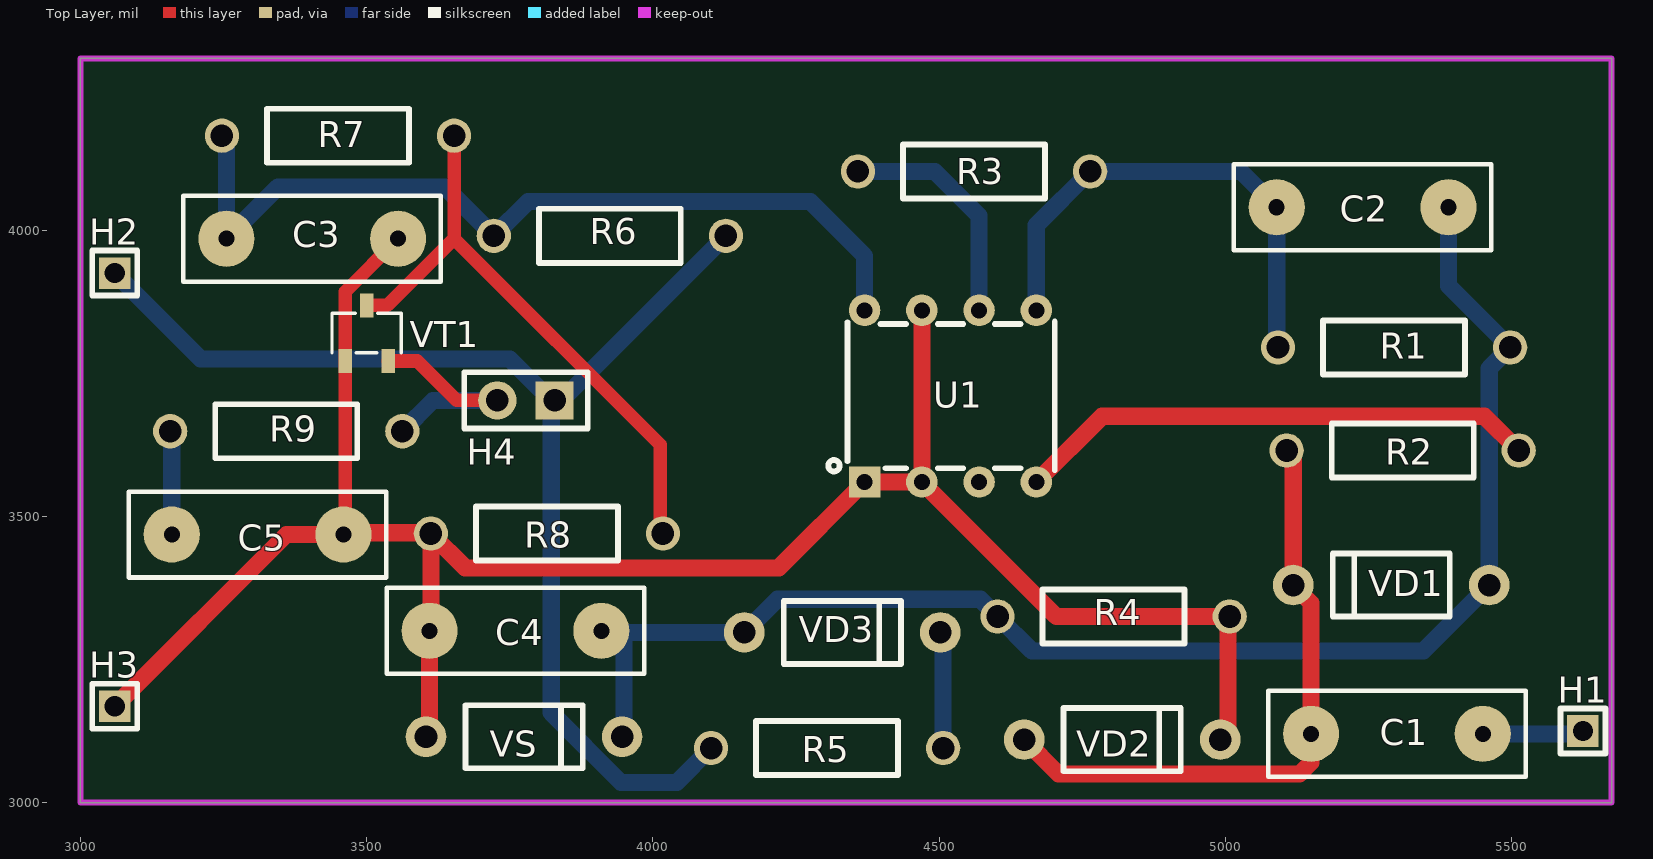
[diagram p0: Top Layer view]
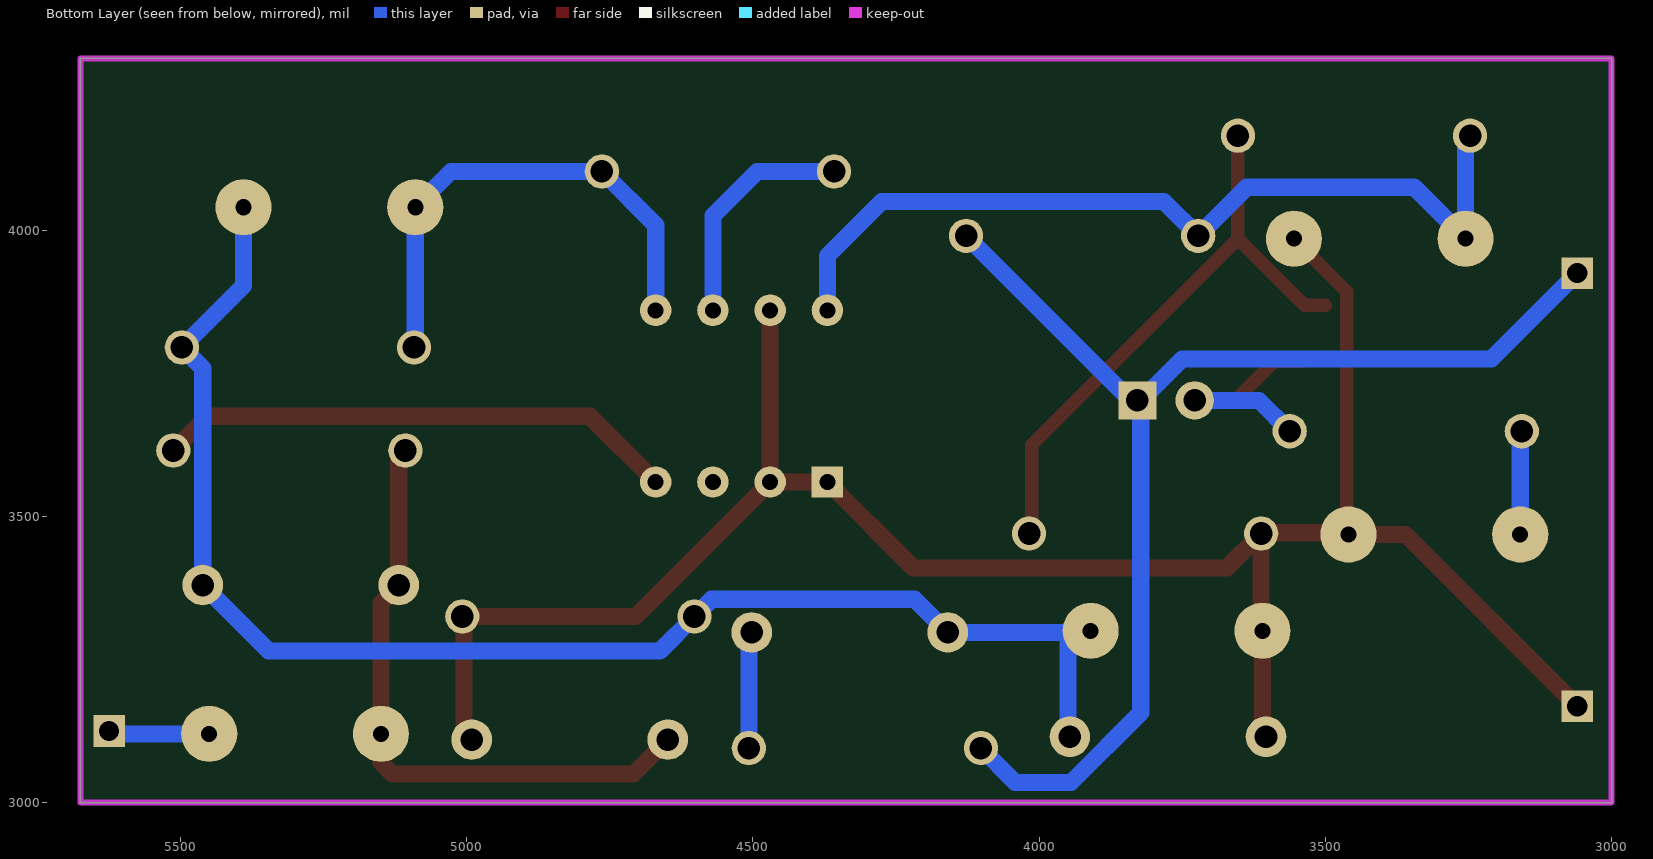
[diagram p1: Bottom Layer view, seen from below]
# Altium PCB MISC75395.pcbdoc
Units mil, origin at the board's own origin, x right, y up, seen from the top; angles counter-clockwise.
Board outline 2675 x 1300 mil, 2 copper layers (Top Layer, Bottom Layer), stack 62.206 mil thick; 24 components, 13 nets, 52 pads, 0 vias.

## Layer stack, top to bottom
Top Solder Mask Layer: solder mask 0.394, Dk 3.3
Top Layer: signal copper 1.379
Dielectric1: surface 59.449, FR4, Dk 4.5
Bottom Layer: signal copper 1.378
Bottom Solder Mask Layer: solder mask 0.394, Dk 3.3

## Board outline
3000,4300 3000,3000 5675,3000 5675,4300

## Design rules (kind name [scope] priority, off if disabled: settings)
BoardOutlineClearance copperThickness2oz_1 [All] p2 off: genericclearance=7.99 ignorepadtopadclearanceinfootprint=FALSE except(0: Arc-SplitContinuation Track-SplitContinuation SMDPad-SplitContinuation THPad-SplitContinuation Via-SplitContinuation Fill-SplitContinuation Region-SplitContinuation Poly-SplitContinuation Text-SplitContinuation Hole-SplitContinuation; 5.98: Arc-CutoutEdge Track-CutoutEdge SMDPad-CutoutEdge THPad-CutoutEdge Via-CutoutEdge Text-CutoutEdge; 6.89: Hole-OutlineEdge Hole-CutoutEdge; 10: Poly-OutlineEdge Poly-CutoutEdge; 11.81: Arc-OutlineEdge Track-OutlineEdge SMDPad-OutlineEdge THPad-OutlineEdge Via-OutlineEdge Fill-OutlineEdge Region-OutlineEdge Text-OutlineEdge Fill-CutoutEdge Region-CutoutEdge)
BoardOutlineClearance Plane_innerPlane_1 [All] p4 off: genericclearance=4.02 ignorepadtopadclearanceinfootprint=FALSE except(0: Arc-SplitContinuation Track-SplitContinuation SMDPad-SplitContinuation THPad-SplitContinuation Via-SplitContinuation Fill-SplitContinuation Region-SplitContinuation Poly-SplitContinuation Text-SplitContinuation Hole-SplitContinuation; 5.98: Arc-CutoutEdge Track-CutoutEdge SMDPad-CutoutEdge THPad-CutoutEdge Via-CutoutEdge Text-CutoutEdge; 6.89: Hole-OutlineEdge Hole-CutoutEdge; 10: Poly-OutlineEdge Poly-CutoutEdge; 11.81: Arc-OutlineEdge Track-OutlineEdge SMDPad-OutlineEdge THPad-OutlineEdge Via-OutlineEdge Fill-OutlineEdge Region-OutlineEdge Text-OutlineEdge Fill-CutoutEdge Region-CutoutEdge)
BoardOutlineClearance Copper_copperRegion_1 [All] p6 off: genericclearance=4.02 ignorepadtopadclearanceinfootprint=FALSE except(0: Arc-SplitContinuation Track-SplitContinuation SMDPad-SplitContinuation THPad-SplitContinuation Via-SplitContinuation Fill-SplitContinuation Region-SplitContinuation Poly-SplitContinuation Text-SplitContinuation Hole-SplitContinuation; 5.98: Arc-CutoutEdge Track-CutoutEdge SMDPad-CutoutEdge THPad-CutoutEdge Via-CutoutEdge Text-CutoutEdge; 6.89: Hole-OutlineEdge Hole-CutoutEdge; 10: Poly-OutlineEdge Poly-CutoutEdge; 11.81: Arc-OutlineEdge Track-OutlineEdge SMDPad-OutlineEdge THPad-OutlineEdge Via-OutlineEdge Fill-OutlineEdge Region-OutlineEdge Text-OutlineEdge Fill-CutoutEdge Region-CutoutEdge)
BoardOutlineClearance copperThickness1oz_1 [All] p8: genericclearance=4.02 ignorepadtopadclearanceinfootprint=FALSE except(0: Arc-SplitContinuation Track-SplitContinuation SMDPad-SplitContinuation THPad-SplitContinuation Via-SplitContinuation Fill-SplitContinuation Region-SplitContinuation Poly-SplitContinuation Text-SplitContinuation Hole-SplitContinuation; 5.98: Arc-CutoutEdge Track-CutoutEdge SMDPad-CutoutEdge THPad-CutoutEdge Via-CutoutEdge Text-CutoutEdge; 6.89: Hole-OutlineEdge Hole-CutoutEdge; 10: Poly-OutlineEdge Poly-CutoutEdge; 11.81: Arc-OutlineEdge Track-OutlineEdge SMDPad-OutlineEdge THPad-OutlineEdge Via-OutlineEdge Fill-OutlineEdge Region-OutlineEdge Text-OutlineEdge Fill-CutoutEdge Region-CutoutEdge)
Clearance copperThickness2oz [All] p1 off: gap=7.99 ignorepadtopadclearanceinfootprint=FALSE except(5.98: SMDPad-Track SMDPad-SMDPad THPad-Track SMDPad-THPad THPad-THPad Track-Via SMDPad-Via THPad-Via Via-Via Fill-SMDPad Region-SMDPad Fill-THPad Region-THPad Fill-Via Region-Via Fill-Fill Fill-Region Region-Region Arc-Track Arc-SMDPad Arc-THPad Arc-Via Fill-Arc Region-Arc Arc-Arc Text-Track SMDPad-Text Text-THPad Text-Via Fill-Text Region-Text Arc-Text Text-Text; 6.89: Hole-Track Hole-SMDPad Hole-THPad Hole-Via Fill-Hole Region-Hole Hole-Arc Hole-Text; 10: Poly-Track Poly-SMDPad Poly-THPad Poly-Via Poly-Fill Poly-Region Poly-Poly Poly-Arc Poly-Text Poly-Hole; 11.81: Fill-Track Region-Track)
Clearance Plane_innerPlane [All] p3 off: gap=4.02 ignorepadtopadclearanceinfootprint=FALSE except(5.98: SMDPad-Track SMDPad-SMDPad THPad-Track SMDPad-THPad THPad-THPad Track-Via SMDPad-Via THPad-Via Via-Via Fill-SMDPad Region-SMDPad Fill-THPad Region-THPad Fill-Via Region-Via Fill-Fill Fill-Region Region-Region Arc-Track Arc-SMDPad Arc-THPad Arc-Via Fill-Arc Region-Arc Arc-Arc Text-Track SMDPad-Text Text-THPad Text-Via Fill-Text Region-Text Arc-Text Text-Text; 6.89: Hole-Track Hole-SMDPad Hole-THPad Hole-Via Fill-Hole Region-Hole Hole-Arc Hole-Text; 10: Poly-Track Poly-SMDPad Poly-THPad Poly-Via Poly-Fill Poly-Region Poly-Poly Poly-Arc Poly-Text Poly-Hole; 11.81: Fill-Track Region-Track)
Clearance Copper_copperRegion [All] p5 off: gap=4.02 ignorepadtopadclearanceinfootprint=FALSE except(5.98: SMDPad-Track SMDPad-SMDPad THPad-Track SMDPad-THPad THPad-THPad Track-Via SMDPad-Via THPad-Via Via-Via Fill-SMDPad Region-SMDPad Fill-THPad Region-THPad Fill-Via Region-Via Fill-Fill Fill-Region Region-Region Arc-Track Arc-SMDPad Arc-THPad Arc-Via Fill-Arc Region-Arc Arc-Arc Text-Track SMDPad-Text Text-THPad Text-Via Fill-Text Region-Text Arc-Text Text-Text; 6.89: Hole-Track Hole-SMDPad Hole-THPad Hole-Via Fill-Hole Region-Hole Hole-Arc Hole-Text; 10: Poly-Track Poly-SMDPad Poly-THPad Poly-Via Poly-Fill Poly-Region Poly-Poly Poly-Arc Poly-Text Poly-Hole; 11.81: Fill-Track Region-Track)
Clearance copperThickness1oz [All] p7: gap=4.02 ignorepadtopadclearanceinfootprint=FALSE except(5.98: SMDPad-Track SMDPad-SMDPad THPad-Track SMDPad-THPad THPad-THPad Track-Via SMDPad-Via THPad-Via Via-Via Fill-SMDPad Region-SMDPad Fill-THPad Region-THPad Fill-Via Region-Via Fill-Fill Fill-Region Region-Region Arc-Track Arc-SMDPad Arc-THPad Arc-Via Fill-Arc Region-Arc Arc-Arc Text-Track SMDPad-Text Text-THPad Text-Via Fill-Text Region-Text Arc-Text Text-Text; 6.89: Hole-Track Hole-SMDPad Hole-THPad Hole-Via Fill-Hole Region-Hole Hole-Arc Hole-Text; 10: Poly-Track Poly-SMDPad Poly-THPad Poly-Via Poly-Fill Poly-Region Poly-Poly Poly-Arc Poly-Text Poly-Hole; 11.81: Fill-Track Region-Track)
DiffPairsRouting differentialPair [All] p1: maxlimit=6 minlimit=6 mostfreqgap=6 toplayer_minwidth=5 toplayer_prefwidth=10 toplayer_maxwidth=100 toplayer_mingap=6 toplayer_prefgap=6 toplayer_maxgap=6 bottomlayer_minwidth=5 bottomlayer_prefwidth=10 bottomlayer_maxwidth=100 bottomlayer_mingap=6 bottomlayer_prefgap=6 bottomlayer_maxgap=6 maxuncoupledlength=10
HoleToHoleClearance otherClearance [All] p1: gap=11.81 allowstackedmicrovias=TRUE
Length netLength [All] p1: minlimit=0 maxlimit=0
PasteMaskExpansion pasteMaskExpansion [All] p1: expansion=0
PlaneConnect innerPlane [All] p1: planeconnectstyle=Relief reliefexpansion=20 reliefentries=4 reliefconductorwidth=10 reliefairgap=10
PolygonConnect copperRegion [All] p1: connectstyle=Relief reliefconductorwidth=10 reliefentries=4 polygonreliefangle="90 Angle" airgapwidth=10 via.connectstyle=Relief via.reliefconductorwidth=10 via.reliefentries=4 via.polygonreliefangle="90 Angle" via.airgapwidth=10
RoutingVias viaSize [All] p1: holewidth=12.01 width=24.02 viastyle="Through Hole" minholewidth=11.81 minwidth=19.68 maxholewidth=248.03 maxwidth=393.7
SolderMaskExpansion solderMaskExpansion [IsVia] p1: expansion=-1000 istentingtop=TRUE
SolderMaskExpansion solderMaskExpansion [All] p2: expansion=2.01 istentingtop=FALSE
Width copperThickness2oz_2 [All] p1 off: maxlimit=100 minlimit=8 preferedwidth=10
Width copperThickness1oz_2 [All] p2: maxlimit=100 minlimit=5 preferedwidth=30

## Components (designator, comment, footprint, x,y, rotation, side; value= is the part's Value field where it differs from the comment)
C1 "" RAD-0.3 5300,3120 r180 top
C2 "" RAD-0.3 5240,4040 r0 top
C3 "" RAD-0.3 3405,3985 r0 top
C4 "" RAD-0.3 3760,3300 r180 top
C5 "" RAD-0.3 3309.61,3468.33 r0 top
H1 "" HDR-TH_1P-V-M_XKB_X4611WV-01I-C28D40 5625,3125 r0 top
H2 "" HDR-TH_1P-V-M_XKB_X4611WV-01I-C28D40 3060,3925 r0 top
H3 "" HDR-TH_1P-V-M_XKB_X4611WV-01I-C28D40 3060,3168.33 r0 top
H4 "" HDR-TH_2P-P2.54-V-F 3778.38,3702.48 r180 top
R1 "1.5M" Res_1/4W 5295,3795 r180 top
R2 "1K" Res_1/4W 5310,3615 r0 top
R3 "20K" Res_1/4W 4561.16,4102.48 r0 top
R4 "360K" Res_1/4W 4805,3325 r0 top
R5 "39K/2W" Res_1/4W 4304.45,3095.18 r180 top
R6 "2M" Res_1/4W 3925,3990 r0 top
R7 "100" Res_1/4W 3450,4165 r0 top
R8 "10K" Res_1/4W 3815,3470 r0 top
R9 "20" Res_1/4W 3359.61,3648.69 r0 top
U1 "" DIP-8_L9.2-W6.6-P2.54-LS7.62-BL 4520,3710 r0 top
VD1 "" DO-41_BD2.4-L4.7-P8.70-D0.9-RD 5290,3380 r0 top
VD2 "1N4148X2" DO-41_BD2.4-L4.7-P8.70-D0.9-RD 4820,3110 r180 top
VD3 "1N4004" DO-41_BD2.4-L4.7-P8.70-D0.9-RD 4331.07,3297.13 r180 top
VS "KEL29VI" DO-41_BD2.4-L4.7-P8.70-D0.9-RD 3775,3115 r180 top
VT1 "97A6" SOT-23-3_L2.9-W1.6-P1.90-LS2.8-BR 3500,3820 r270 top

## Footprints (in the part's own frame and the unit in brackets; to place one, negate y for a bottom-side part, rotate by r counter-clockwise, add the part's x,y. Pads: shape width x height; smd on the part's side, far side on the other; paste and mask are expansions set on the pad)
DIP-8_L9.2-W6.6-P2.54-LS7.62-BL [mil]
  rect 55x55 hole 28: 1(-150,-150)
  round 55 hole 28: 2(-50,-150) 3(50,-150) 4(150,-150) 5(150,150) 6(50,150) 7(-50,150) 8(-150,150)
  silkscreen extent -214,-132 182,130
DO-41_BD2.4-L4.7-P8.70-D0.9-RD [mm]
  round 1.8 hole 1: 1(-4.35,0) 3(4.35,0)
  silkscreen extent -2.6,-1.4 2.6,1.4
HDR-TH_1P-V-M_XKB_X4611WV-01I-C28D40 [mm]
  rect 1.4x1.4 hole 0.9: 1(0,0)
  silkscreen extent -1,-1 1,1
HDR-TH_2P-P2.54-V-F [mm]
  rect 1.7x1.7 hole 1: 1(-1.27,0)
  round 1.7 hole 1: 2(1.27,0)
  silkscreen extent -2.74,-1.25 2.74,1.25
RAD-0.3 [mil]
  round 98 hole 28: 1(150,0) 2(-150,0)
  silkscreen extent -225,-75 225,75
Res_1/4W [mil]
  round 60 hole 39.37 paste+0 mask+2: 1(-202.76,0) 2(202.76,0)
  silkscreen extent -124,-47 124,47
SOT-23-3_L2.9-W1.6-P1.90-LS2.8-BR [mm]
  rect 1.07x0.6 smd: 1(1.235,-0.95) 2(1.235,0.95) 3(-1.235,0)
  silkscreen extent -0.88,-1.54 0.88,1.54

## Nets (pads, with @x,y where several pads share a name; then routed paths per layer and width w, separated by ;. In a path a pad name is that pad's centre, name@x,y a point inside that pad or via, vN(x,y) a via of type N, cw(c..) or ccw(c..) an arc to the next point about the centre after c; other vN are vias at no path point)
$1N1: C1.2 H1.1 | length 177.1
  Bottom Layer w30: C1.2 5620,3120 H1.1
$1N2: C1.1 R2.1 VD1.1 VD2.3 | length 1097.1
  Top Layer w30: VD2.3 4708.74,3050 5130,3050 5150,3070 C1.1 5150,3348.74 VD1.1 5118.74,3603.5 R2.1
$1N4: C3.1 C4.1 C5.1 H3.1 R4.2 R8.1 U1.1 U1.2 U1.7 VD2.1 VS.3 VT1.1 | length 3689.3
  Top Layer w23.62: C5.1 3462.6,3471.38 VT1.1 3462.6,3892.6 C3.1
  Top Layer w30: H3.1 3360,3468.33 C5.1 ; C5.1@3462.6,3471.38 3610.86,3471.38 R8.1 ; VS.3 3610,3121.26 C4.1 3612.24,3302.24 R8.1 ; U1.7 U1.2 ; VD2.1 5005,3123.74 R4.2@5005,3325 ; R4.2 R4.2@5005,3325 ; R8.1 3672.24,3410 4220,3410 U1.1 U1.2 ; U1.2 4705,3325 R4.2@5005,3325
$1N8: C2.2 R1.2 R3.2 U1.5 | length 879.3
  Bottom Layer w30: U1.5 4670,4008.57 R3.2 5027.52,4102.48 C2.2 5090,3797.24 R1.2
$1N13: H2.1 H4.1 R5.2 R6.2 | length 2179
  Bottom Layer w30: H2.1 3210,3775 3750,3775 H4.1@3822.52,3702.48 ; R5.2 4041.69,3035.18 3944.39,3035.18 3822.52,3157.04 H4.1@3822.52,3702.48 ; R6.2 3840.24,3702.48 H4.1 H4.1@3822.52,3702.48
$1N14: R5.1 VD3.1 | length 204
  Bottom Layer w30: VD3.1 4507.21,3292.24 R5.1
$1N16: C3.2 R6.1 R7.1 U1.8 | length 1529.9
  Bottom Layer w30: R7.1 3255,4157.24 C3.2 3345,4075 3637.24,4075 R6.1 3782.24,4050 4275,4050 4370,3955 U1.8
$1N19: C5.2 R9.1 | length 181.5
  Bottom Layer w30: R9.1@3156.85,3648.69 3159.61,3645.93 C5.2
$1N1376: H4.2 R9.2 VT1.2 | length 407.8
  Top Layer w23.62: VT1.2 3588.62,3771.38 3657.52,3702.48 H4.2
  Bottom Layer w30: R9.2 3616.16,3702.48 H4.2
$1N1401: C2.1 C4.2 R1.1 R4.1 VD1.3 VD3.3 VS.1 | length 2564.7
  Bottom Layer w30: C4.2 3912.87,3297.13 C4.2@3949.81,3297.13 ; VS.1 3949.81,3118.55 C4.2@3949.81,3297.13 ; C2.1 5390,3902.76 R1.1 5461.26,3758.5 VD1.3 5346.26,3265 4662.24,3265 R4.1 4572.24,3355 4217.68,3355 VD3.3 C4.2@3949.81,3297.13
$1N1405: R7.2 R8.2 VT1.3 | length 1047.2
  Top Layer w23.62: VT1.3 3536.39,3868.62 3652.76,3985 ; R7.2 3652.76,3985 ; R8.2 4012.76,3475 4012.76,3625 3652.76,3985
$1N1991: R2.2 U1.4 | length 915.2
  Top Layer w30: U1.4 4785,3675 5452.76,3675 R2.2
$1N2847: R3.1 U1.6 | length 408.7
  Bottom Layer w30: R3.1 4492.52,4102.48 4570,4025 U1.6
pads on no net: U1.3

## Keep-outs
Board Outline Layer:
  the board outline again, w10